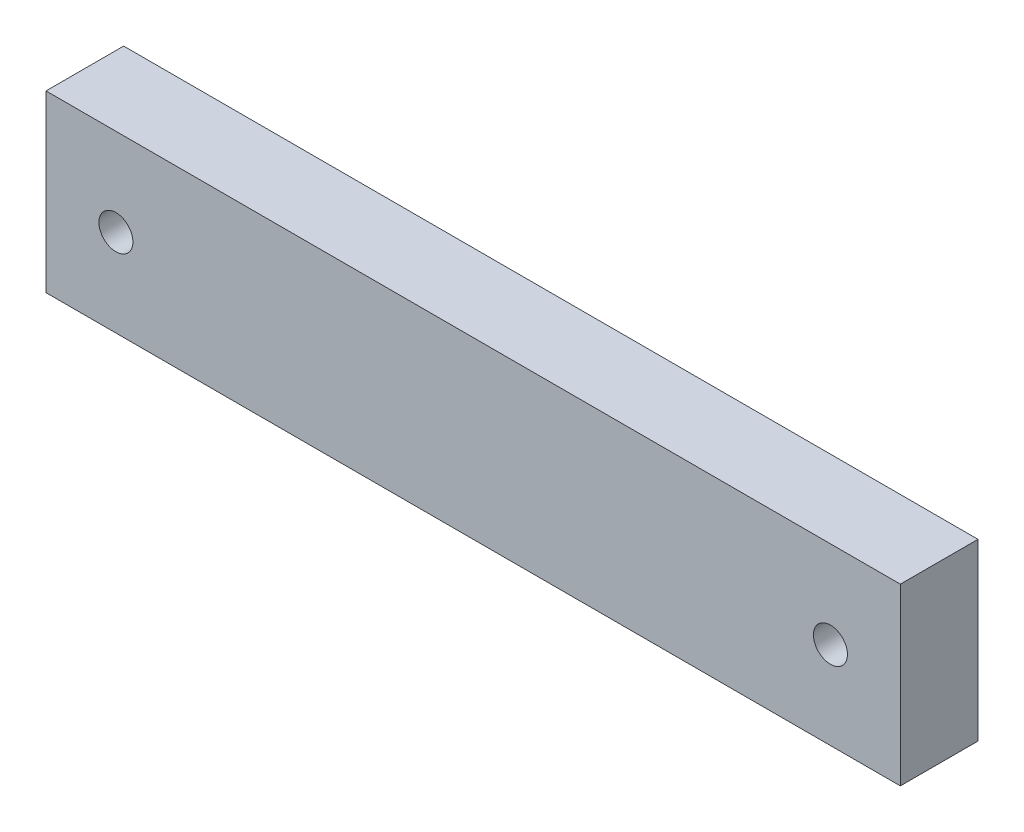
from build123d import *

# Parameters (mm, degrees)
SKETCH1_W           = 440
SKETCH1_H           = 90
BOSS_EXTRUDE1_DEPTH = 40
M20_TAPPED_HOLE1_D  = 17.5


with BuildPart() as part:
    # Sketch1 → Boss-Extrude1 (new body)
    with BuildSketch(Plane.XY):
        with Locations((220, 45)):
            Rectangle(SKETCH1_W, SKETCH1_H)
    extrude(amount=BOSS_EXTRUDE1_DEPTH)

    # M20 Tapped Hole1 (through all)
    with Locations(Plane.XY.offset(40)):
        with Locations((36, 45), (404, 45)):
            Hole(M20_TAPPED_HOLE1_D / 2)


solid = part.part
